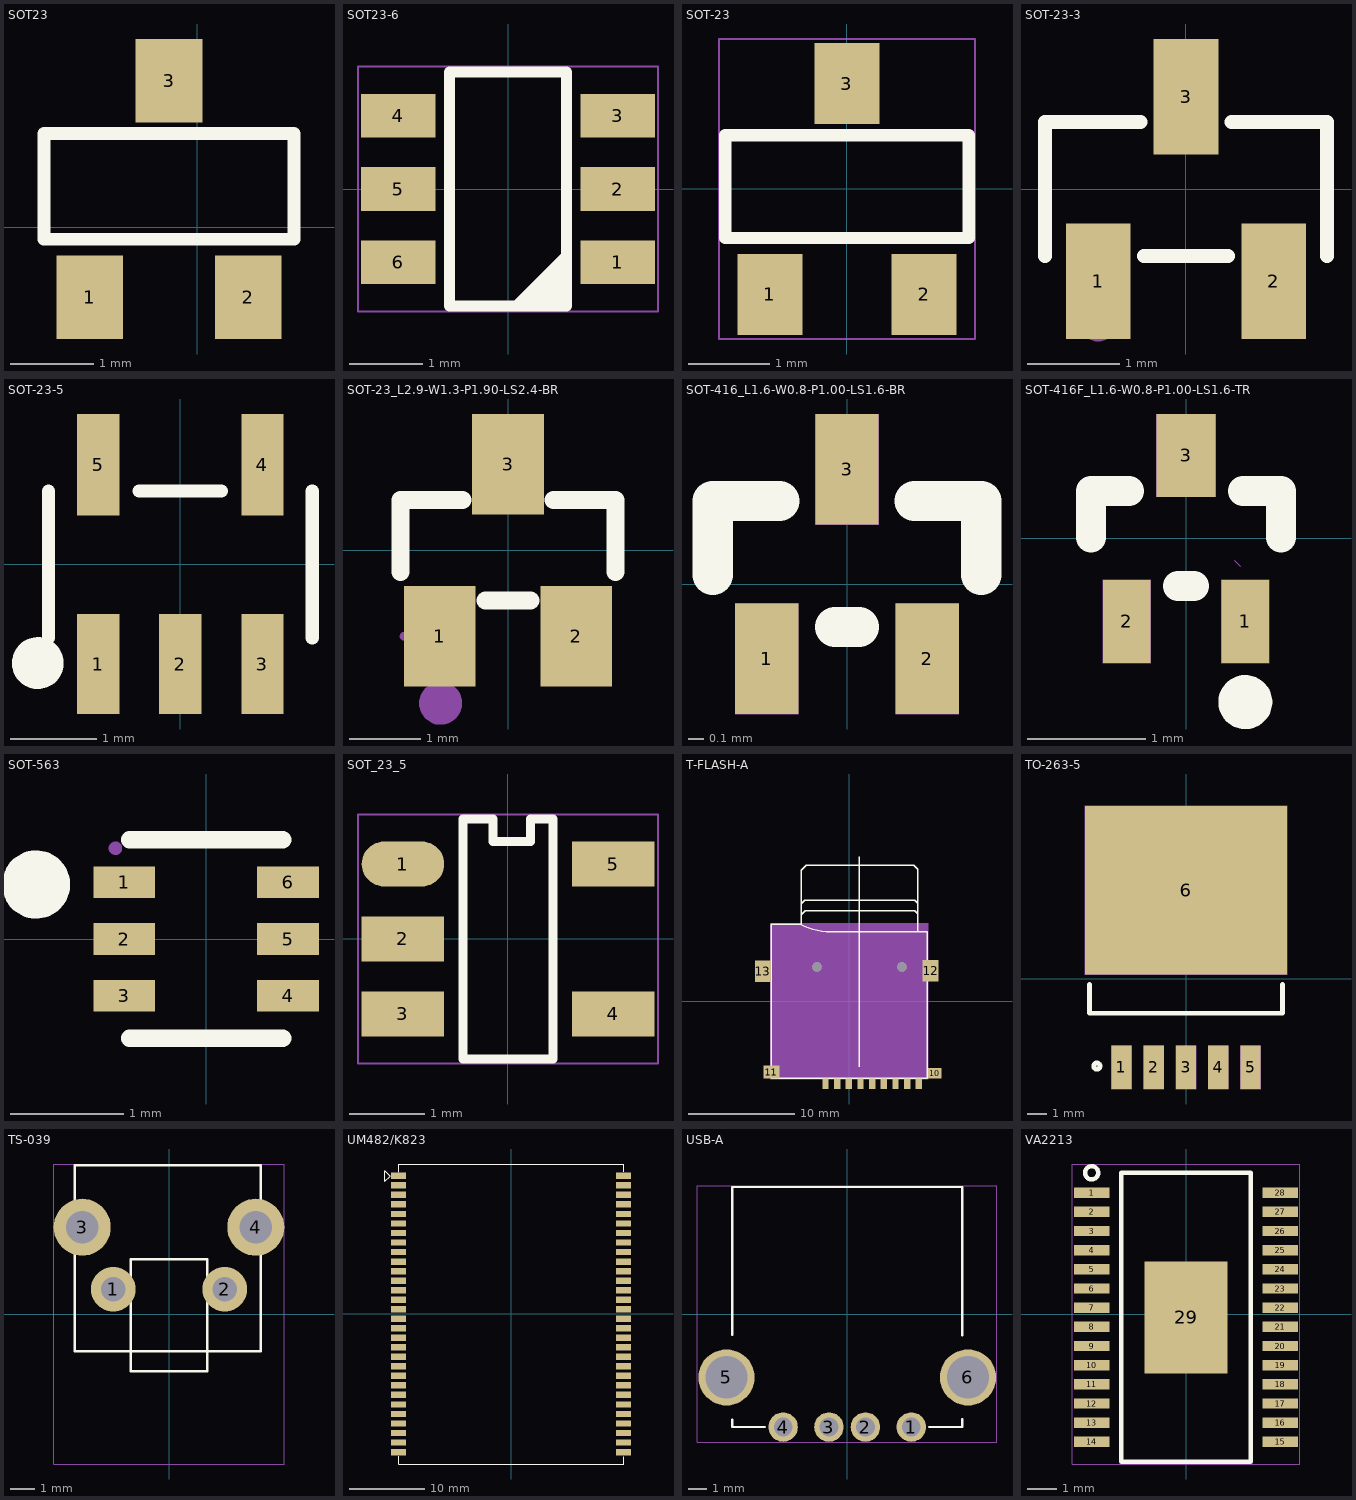
[diagram p0: the footprints below, top view; thin cyan lines are the x and y axes]
# Altium footprint library MISC84456-5.PcbLib: 85 footprints (part 5 of 6)
Each footprint in its own frame and in the unit in brackets; x right, y up, seen from the top. Pads: shape width x height; smd on the part's side, far side on the other; paste and mask are expansions set on the pad; w line width, h text height; cw(c..) or ccw(c..) is an arc to the next point about the centre after c.

## SOT23 [mil] "SOT23"
pads (3):
  rect 31.5x39.4 smd: 1(-50.85,-33.2) 2(23.95,-33.2) 3(-13.45,69.2)
Top Overlay:
  lines w6: -72.55,-5.8 45.65,-5.8 45.65,44.2 -72.55,44.2 -72.55,-5.8
  text ".Designator" at -55.77,-84.36 h23.62
Mechanical 7:
  text "3" at -13.45,59.2 h25
  text "2" at 23.95,-43.2 h25
  text "1" at -50.85,-43.2 h25
Mechanical 9:
  text "PESD1CAN" at -3.61,-36.13 h13.78

## SOT23-6 [mil] "SOT23-6"
pads (6):
  rect 40x23.6 smd: 1(59.1,-39.4) 2(59.1,0) 3(59.1,39.4) 4(-59.1,39.4) 5(-59.1,0) 6(-59.1,-39.4)
Top Overlay:
  lines w6: 5.1,-62.4 31.1,-36.4 ; 24.1,-61.4 31.1,-54.4 ; -31.5,-63 31.5,-63 31.5,63 -31.5,63 -31.5,-63
  lines w8: 14.3,-58.2 27.3,-45.2 ; 17.1,-61.4 30.1,-48.4
Mechanical 7:
  text "2" at 49.1,0 h25
  text "5" at -69.1,0 h25
  text "4" at -69.1,39.4 h25
  text "3" at 49.1,39.4 h25
  text "6" at -69.1,-39.4 h25
  text "1" at 49.1,-39.4 h25
Mechanical 8:
  lines w1: -80.7,-66 -80.7,66 80.7,66 80.7,-66 -80.7,-66
Mechanical 9:
  text ".Designator" at -27.56,-8.86 h13.78
  text "SY8113B" at -55.12,-3.94 h13.78

## SOT-23 [mm] "SOT-23"
pads (3):
  rect 0.8x1 smd: 1(-0.95,-1.3) 2(0.95,-1.3) 3(0,1.3)
Top Overlay:
  lines w0.152: -1.5,-0.605 -1.5,0.665 1.5,0.665 1.5,-0.605 -1.5,-0.605
Mechanical 7:
  text "2" at 0.696,-1.3 h0.64
  text "3" at -0.254,1.3 h0.64
  text "1" at -1.204,-1.3 h0.64
Mechanical 8:
  lines w0.025: -1.576,-1.85 -1.576,1.85 1.576,1.85 1.576,-1.85 -1.576,-1.85
Mechanical 9:
  text ".Designator" at -0.075,0.45 h0.35
  text "MMBT3904" at -1.35,-0.025 h0.35

## SOT-23-3 [mm]
pads (3):
  rect 0.7x1.25 smd: 1(-0.95,-1) 2(0.95,-1) 3(0,1)
Top Overlay:
  lines w0.152: -1.526,-0.726 -1.526,0.726 -0.495,0.726 ; -0.455,-0.726 0.455,-0.726 ; 0.495,0.726 1.526,0.726 1.526,-0.726
Mechanical 5:
  region: -1.165,-0.85 -0.735,-0.85 -0.735,-1.15 -1.165,-1.15
  pour cut-out: -1.165,-0.64 -0.735,-0.64 -0.735,-0.86 -1.165,-0.86
  region: 0.735,-0.85 1.165,-0.85 1.165,-1.15 0.735,-1.15
  pour cut-out: 0.735,-0.64 1.165,-0.64 1.165,-0.86 0.735,-0.86
  region: -0.215,0.85 0.215,0.85 0.215,1.15 -0.215,1.15
  pour cut-out: -0.215,0.86 0.215,0.86 0.215,0.64 -0.215,0.64
Mechanical 15:
  circle w0.2: c-0.95,-1.45 r0.1

## SOT-23-5 [mm]
pads (5):
  rect 0.49x1.157 smd: 1(-0.95,-1.154) 2(0,-1.154) 3(0.95,-1.154)
  rect 0.49x1.175 smd: 4(0.95,1.154) 5(-0.95,1.154)
Top Overlay:
  circle w0.3: c-1.651,-1.143 r0.15
  lines w0.152: -1.526,-0.851 -1.526,0.851 ; -0.476,0.851 0.476,0.851 ; 1.526,-0.851 1.526,0.851
Mechanical 5:
  region: -0.175,-1.4 -0.175,-1 0.175,-1 0.175,-1.4
  pour cut-out: -0.175,-1.01 -0.175,-0.74 0.175,-0.74 0.175,-1.01
  region: 0.775,-1.4 0.775,-1 1.125,-1 1.125,-1.4
  pour cut-out: 0.775,-1.01 0.775,-0.74 1.125,-0.74 1.125,-1.01
  region: 0.775,1 0.775,1.4 1.125,1.4 1.125,1
  pour cut-out: 0.775,0.74 0.775,1.01 1.125,1.01 1.125,0.74
  region: -1.125,1 -1.125,1.4 -0.775,1.4 -0.775,1
  pour cut-out: -1.125,0.74 -1.125,1.01 -0.775,1.01 -0.775,0.74

## SOT-23_L2.9-W1.3-P1.90-LS2.4-BR [mm]
pads (3):
  rect 1x1.4 smd: 1(-0.95,-1.2) 2(0.95,-1.2) 3(0,1.2)
Top Overlay:
  lines w0.254: -1.5,-0.3 -1.5,0.7 -0.636,0.7 ; -0.314,-0.7 0.314,-0.7 ; 0.636,0.7 1.5,0.7 1.5,-0.3
Mechanical 5:
  pour cut-out: -0.242,1.01 0.243,1.01 0.243,0.64 -0.242,0.64
  region: -0.242,1.2 0.243,1.2 0.243,1 -0.242,1
  pour cut-out: 0.708,-0.64 1.193,-0.64 1.193,-1.01 0.708,-1.01
  region: 0.708,-1 1.193,-1 1.193,-1.2 0.708,-1.2
  pour cut-out: -1.192,-0.64 -0.707,-0.64 -0.707,-1.01 -1.192,-1.01
  region: -1.192,-1 -0.707,-1 -0.707,-1.2 -1.192,-1.2
Mechanical 6:
  circle w0.06: c-1.45,-1.2 r0.03
Mechanical 15:
  circle w0.3: c-0.94,-2.134 r0.15

## SOT-416_L1.6-W0.8-P1.00-LS1.6-BR [mm]
pads (3):
  rect 0.4x0.7 smd: 1(-0.508,-0.473) 2(0.508,-0.473) 3(0,0.727)
Top Overlay:
  lines w0.254: -0.85,0.059 -0.85,0.527 -0.428,0.527 ; -0.077,-0.273 0.077,-0.273 ; 0.428,0.527 0.85,0.527 0.85,0.059
Mechanical 5:
  region: 0.2,1.077 0.2,0.377 -0.2,0.377 -0.2,1.077
  region: 0.708,-0.123 0.708,-0.823 0.308,-0.823 0.308,-0.123
  region: -0.308,-0.123 -0.308,-0.823 -0.708,-0.823 -0.708,-0.123

## SOT-416F_L1.6-W0.8-P1.00-LS1.6-TR [mm]
pads (3):
  rect 0.4x0.7 smd: 1(0.5,-0.7) 2(-0.5,-0.7)
  rect 0.5x0.7 smd: 3(0,0.7)
Top Overlay:
  circle w0.254: c0.5,-1.38 r0.101
  lines w0.254: -0.8,0.009 -0.8,0.4 -0.481,0.4 ; -0.068,-0.4 0.068,-0.4 ; 0.481,0.4 0.8,0.4 0.8,0.009
Mechanical 5:
  region: -0.299,-0.349 -0.299,-1.05 -0.701,-1.05 -0.701,-0.349
  region: 0.701,-0.349 0.701,-1.05 0.299,-1.05 0.299,-0.349
  region: 0.25,1.05 0.25,0.35 -0.25,0.35 -0.25,1.05
Mechanical 15:
  lines w0.003: 0.408,-0.184 0.459,-0.235

## SOT-563 [mm]
pads (6):
  rect 0.545x0.28 smd: 1(-0.723,0.5) 2(-0.723,0) 3(-0.723,-0.5) 4(0.723,-0.5) 5(0.723,0) 6(0.723,0.5)
Top Overlay:
  circle w0.3: c-1.5,0.481 r0.15
  lines w0.152: -0.676,-0.876 0.676,-0.876 ; -0.676,0.876 0.676,0.876
Mechanical 5:
  region: -0.586,0.612 -0.586,0.387 -0.811,0.387 -0.811,0.612
  region: -0.586,0.112 -0.586,-0.112 -0.811,-0.112 -0.811,0.112
  region: -0.586,-0.388 -0.586,-0.613 -0.811,-0.613 -0.811,-0.388
  region: 0.811,-0.388 0.811,-0.613 0.586,-0.613 0.586,-0.388
  region: 0.811,0.112 0.811,-0.112 0.586,-0.112 0.586,0.112
  region: 0.811,0.612 0.811,0.387 0.586,0.387 0.586,0.612
Mechanical 6:
  circle w0.06: c-0.8,0.8 r0.03

## SOT_23_5 [mm] "SOT_23_5"
pads (5):
  oval 1.1x0.6 smd: 1(-1.4,1)
  rect 1.1x0.6 smd: 2(-1.4,0) 3(-1.4,-1) 4(1.4,-1) 5(1.4,1)
Top Overlay:
  lines w0.12: -0.6,-1.6 0.6,-1.6 0.6,1.6 0.3,1.6 0.3,1.3 -0.2,1.3 -0.2,1.6 -0.6,1.6 -0.6,-1.6
Mechanical 7:
  text "4" at 1.146,-1 h0.64
  text "3" at -1.654,-1 h0.64
  text "5" at 1.146,1 h0.64
  text "1" at -1.654,1 h0.64
  text "2" at -1.654,0 h0.64
Mechanical 8:
  lines w0.025: -2,-1.66 2,-1.66 2,1.66 -2,1.66 -2,-1.66
Mechanical 9:
  text "LPW5206" at -1.4,-0.225 h0.35
  text ".Designator" at -0.425,0.6 h0.35

## T-FLASH-A [mil] "T-FLASH-A"
pads (15):
  rect 23.6x39.4 smd: 1(-88.57,-305.13) 2(-45.27,-305.13) 3(-1.97,-305.13) 4(41.33,-305.13) 5(84.63,-305.13) 6(127.93,-305.13) 7(171.23,-305.13) 8(214.53,-305.13) 9(257.83,-305.13)
  rect 51.2x39.4 smd: 10(316.93,-265.73)
  rect 59.1x47.2 smd: 11(-289.37,-261.83)
  rect 59.1x78.7 smd: 12(301.23,114.19) 13(-320.87,112.17)
  round 35 hole 35: " "(-120.07,127.97) " "(194.93,127.97)
Top Overlay:
  lines w5: -179.17,285.47 -179.17,486.27 -159.47,505.87 238.23,505.87 253.93,490.17 253.93,257.87 ; -179.17,320.87 -163.37,336.57 242.13,336.57 253.93,324.77 ; -178.17,363.17 -165.37,375.97 242.13,375.97 253.93,364.17 ; 37.43,-242.13 37.43,537.37 ; -289.37,-285.43 289.33,-285.43 289.33,257.87 -53.17,257.87 cw(c-64.75,522.83) -183.07,285.47 -289.37,285.47 -289.37,-285.43
Mechanical 7:
  text "3" at -11.97,-305.13 h25
  text "9" at 247.83,-305.13 h25
  text "2" at -55.27,-305.13 h25
  text "8" at 204.53,-305.13 h25
  text "1" at -98.57,-305.13 h25
  text "4" at 31.33,-305.13 h25
  text "7" at 161.23,-305.13 h25
  text "5" at 74.63,-305.13 h25
  text "13" at -340.87,112.17 h25
  text "11" at -309.37,-261.83 h25
  text "10" at 296.93,-265.73 h25
  text "12" at 281.23,114.19 h25
  text "6" at 117.93,-305.13 h25
Mechanical 8:
  region: -293.31,289.37 -293.31,-289.37 293.31,-289.37 293.31,289.37
Mechanical 9:
  text ".Designator" at -49.21,170.28 h13.78

## TO-263-5 [mil]
pads (6):
  rect 42.1x90 smd: 1(-134,-183.77) 2(-67,-183.77) 3(0,-183.77) 4(67,-183.77) 5(134,-183.77)
  rect 419.68x350 smd: 6(0,183.77)
Top Overlay:
  circle w10: c-185,-181.27 r6.5
  lines w10: -200,-11.27 -200,-71.77 200,-71.77 200,-11.27
Mechanical 5:
  region: -155.05,-228.77 -155.05,-138.77 -112.95,-138.77 -112.95,-228.77
  region: -21.05,-228.77 -21.05,-138.77 21.05,-138.77 21.05,-228.77
  region: -88.05,-228.77 -88.05,-138.77 -45.95,-138.77 -45.95,-228.77
  region: 45.95,-228.77 45.95,-138.77 88.05,-138.77 88.05,-228.77
  region: 112.95,-228.77 112.95,-138.77 155.05,-138.77 155.05,-228.77
  region: -209.84,8.77 -209.84,358.77 209.84,358.77 209.84,8.77
Mechanical 15:
  lines w0.1: -19.75,65.77 -17.75,63.77

## TS-039 [mm] "TS-039"
pads (4):
  round 1.8 hole 1: 1(-2.25,1) 2(2.25,1)
  round 2.3 hole 1.3: 3(-3.5,3.5) 4(3.5,3.5)
Top Overlay:
  lines w0.1: -3.8,-1.5 -3.8,6 3.7,6 3.7,-1.5 -3.8,-1.5 ; -1.55,-2.3 1.55,-2.3 1.55,2.2 -0.05,2.2 -1.55,2.2 -1.55,-2.3
Mechanical 7:
  text "3" at -3.564,3.5 h0.08
  text "4" at 3.436,3.5 h0.08
  text "2" at 2.186,1 h0.08
  text "1" at -2.314,1 h0.08
Mechanical 8:
  lines w0.025: -4.65,-6.05 -4.65,6.05 4.65,6.05 4.65,-6.05 -4.65,-6.05
Mechanical 9:
  text ".Designator" at -0.5,2.8 h0.35
  text "RESET" at -0.825,2.575 h0.35

## UM482/K823 [mm]
pads (60):
  rect 2.01x0.85 smd: 1(-15,18.415) 2(-15,17.145) 3(-15,15.875) 4(-15,14.605) 5(-15,13.335) 6(-15,12.065) 7(-15,10.795) 8(-15,9.525) 9(-15,8.255) 10(-15,6.985) 11(-15,5.715) 12(-15,4.445) 13(-15,3.175) 14(-15,1.905) 15(-15,0.635) 16(-15,-0.635) 17(-15,-1.905) 18(-15,-3.175) 19(-15,-4.445) 20(-15,-5.715) 21(-15,-6.985) 22(-15,-8.255) 23(-15,-9.525) 24(-15,-10.795) 25(-15,-12.065) 26(-15,-13.335) 27(-15,-14.605) 28(-15,-15.875) 29(-15,-17.145) 30(-15,-18.415) 31(15,-18.415) 32(15,-17.145) 33(15,-15.875) 34(15,-14.605) 35(15,-13.335) 36(15,-12.065) 37(15,-10.795) 38(15,-9.525) 39(15,-8.255) 40(15,-6.985) 41(15,-5.715) 42(15,-4.445) 43(15,-3.175) 44(15,-1.905) 45(15,-0.635) 46(15,0.635) 47(15,1.905) 48(15,3.175) 49(15,4.445) 50(15,5.715) 51(15,6.985) 52(15,8.255) 53(15,9.525) 54(15,10.795) 55(15,12.065) 56(15,13.335) 57(15,14.605) 58(15,15.875) 59(15,17.145) 60(15,18.415)
Top Overlay:
  lines w0.1: -15,-18.95 -15,-20.005 15,-20.005 15,-19.01 ; -15,18.92 -15,19.995 15,19.995 15,18.93 ; -16.81,17.69 -16.13,18.37 -16.13,18.44 -16.14,18.44 -16.81,19.11 -16.81,17.69

## USB-A [mil] "USB-A"
pads (6):
  round 62.99 hole 40: 1(137.5,-241.5) 2(39.5,-241.5) 3(-38.5,-241.5) 4(-136.5,-241.5)
  round 120 hole 90.55: 5(-257.5,-135.5) 6(258.5,-135.5)
Top Overlay:
  lines w5: -245.5,-225.5 -245.5,-241.5 -175.5,-241.5 ; -245.5,-44.5 -245.5,271.5 246.5,271.5 246.5,-45.5 ; 175.5,-241.5 246.5,-241.5 246.5,-224.5
Mechanical 7:
  text "4" at -138.9,-241.5 h3
  text "1" at 135.1,-241.5 h3
  text "6" at 256.1,-135.5 h3
  text "5" at -259.9,-135.5 h3
  text "3" at -40.9,-241.5 h3
  text "2" at 37.1,-241.5 h3
Mechanical 8:
  lines w1: -320.5,-274.5 -320.5,274.5 320.5,274.5 320.5,-274.5 -320.5,-274.5

## VA2213 [mm] "VA2213"
pads (29):
  rect 1.2x0.35 smd: 1(-3.2,4.113) 2(-3.2,3.463) 3(-3.2,2.813) 4(-3.2,2.163) 5(-3.2,1.513) 6(-3.2,0.863) 7(-3.2,0.213) 8(-3.2,-0.437) 9(-3.2,-1.087) 10(-3.2,-1.737) 11(-3.2,-2.387) 12(-3.2,-3.037) 13(-3.2,-3.687) 14(-3.2,-4.337) 15(3.2,-4.337) 16(3.2,-3.687) 17(3.2,-3.037) 18(3.2,-2.387) 19(3.2,-1.737) 20(3.2,-1.087) 21(3.2,-0.437) 22(3.2,0.213) 23(3.2,0.863) 24(3.2,1.513) 25(3.2,2.163) 26(3.2,2.813) 27(3.2,3.463) 28(3.2,4.113)
  rect 2.8x3.8 smd: 29(0,-0.112)
Top Overlay:
  circle w0.15: c-3.2,4.788 r0.224
  lines w0.025: -2.15,-4.962 -2.15,4.738 2.15,4.738 2.15,-4.962 -2.15,-4.962
  lines w0.15: -2.2,-5.012 -2.2,4.788 2.2,4.788 2.2,4.588 2.2,-5.012 -2.2,-5.012
  text ".Designator" at -0.8,5.238 h0.6
Mechanical 7:
  text "19" at 2.794,-1.737 h0.51
  text "14" at -3.606,-4.337 h0.51
  text "24" at 2.794,1.513 h0.51
  text "29" at -2.083,-0.112 h0.51
  text "8" at -3.403,-0.437 h0.51
  text "28" at 2.794,4.113 h0.51
  text "27" at 2.794,3.463 h0.51
  text "15" at 2.794,-4.337 h0.51
  text "16" at 2.794,-3.687 h0.51
  text "4" at -3.403,2.163 h0.51
  text "11" at -3.606,-2.387 h0.51
  text "23" at 2.794,0.863 h0.51
  text "17" at 2.794,-3.037 h0.51
  text "13" at -3.606,-3.687 h0.51
  text "7" at -3.403,0.213 h0.51
  text "2" at -3.403,3.463 h0.51
  text "1" at -3.403,4.113 h0.51
  text "25" at 2.794,2.163 h0.51
  text "5" at -3.403,1.513 h0.51
  text "6" at -3.403,0.863 h0.51
  text "20" at 2.794,-1.087 h0.51
  text "26" at 2.794,2.813 h0.51
  text "3" at -3.403,2.813 h0.51
  text "9" at -3.403,-1.087 h0.51
  text "21" at 2.794,-0.437 h0.51
  text "22" at 2.794,0.213 h0.51
  text "12" at -3.606,-3.037 h0.51
  text "10" at -3.606,-1.737 h0.51
  text "18" at 2.794,-2.387 h0.51
Mechanical 8:
  lines w0.025: -3.85,-5.087 -3.85,5.087 3.85,5.087 3.85,-5.087 -3.85,-5.087